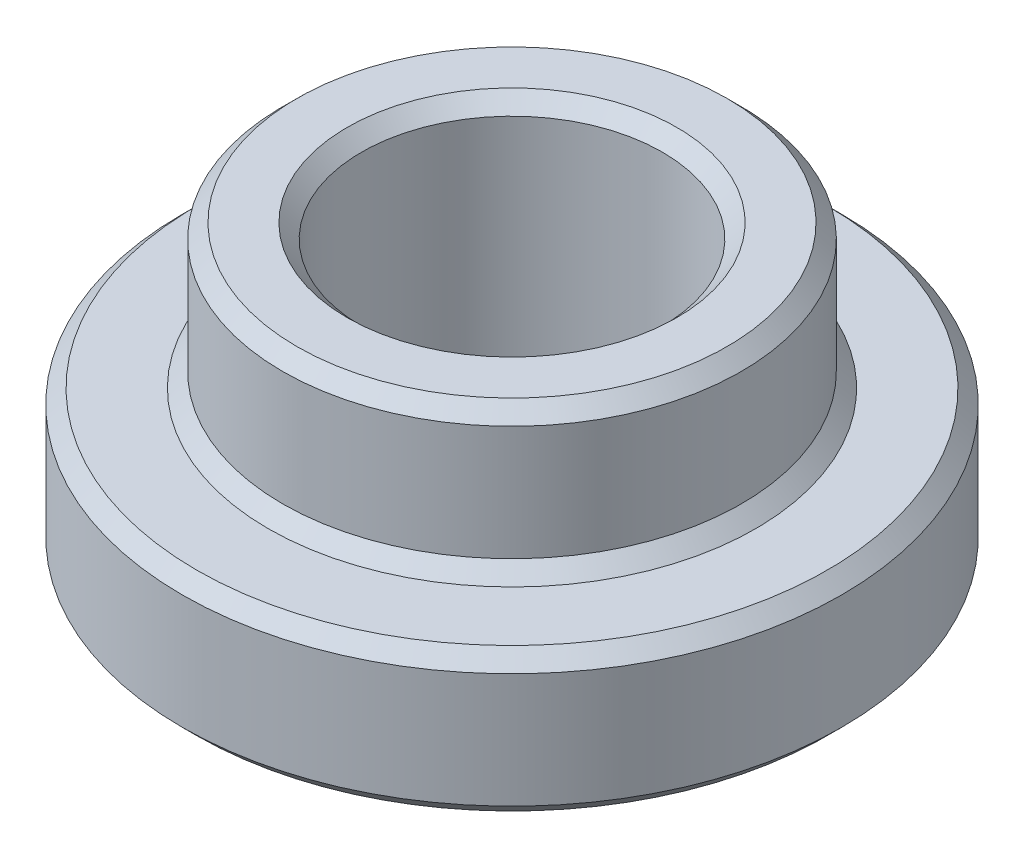
SolidWorks part; units mm, degrees
ref_plane "Front Plane" through (0, 0, 0) normal (0, 0, 1) x (1, 0, 0)
ref_plane "Top Plane" through (0, 0, 0) normal (0, 1, 0) x (1, 0, 0)
ref_plane "Right Plane" through (0, 0, 0) normal (1, 0, 0) x (0, 0, -1)
other "Configuration Table"
sketch "Sketch1" plane through (0, 0, 0) normal (0, 1, 0) x (1, 0, 0)
  circle A0 centre (0, 0) radius 23
  dimension "D1" = 46
extrude "Boss-Extrude1" add sketch "Sketch1" along normal blind 10
sketch "Sketch2" plane through (0, 10, 0) normal (0, 1, 0) x (1, 0, 0)
  circle A0 centre (0, 0) radius 16
  dimension "D1" = 32
extrude "Boss-Extrude2" add sketch "Sketch2" along normal blind 10 contours A0
sketch "Sketch3" plane through (0, 20, 0) normal (0, 1, 0) x (1, 0, 0)
  circle A0 centre (0, 0) radius 10.5
  dimension "D1" = 21
extrude "Cut-Extrude1" cut sketch "Sketch3" against normal blind 20
cosmetic thread "Cosmetic Thread1" parameters "D2"=24
chamfer "Chamfer1" distance 1 angle 45 5 edges at (0, 0, 23) (0, 10, 23) (0, 10, 16) (0, 20, 16) (0, 20, 10.5)
chamfer "Chamfer2" distance 1 angle 45 1 edges at (0, 0, 10.5)
